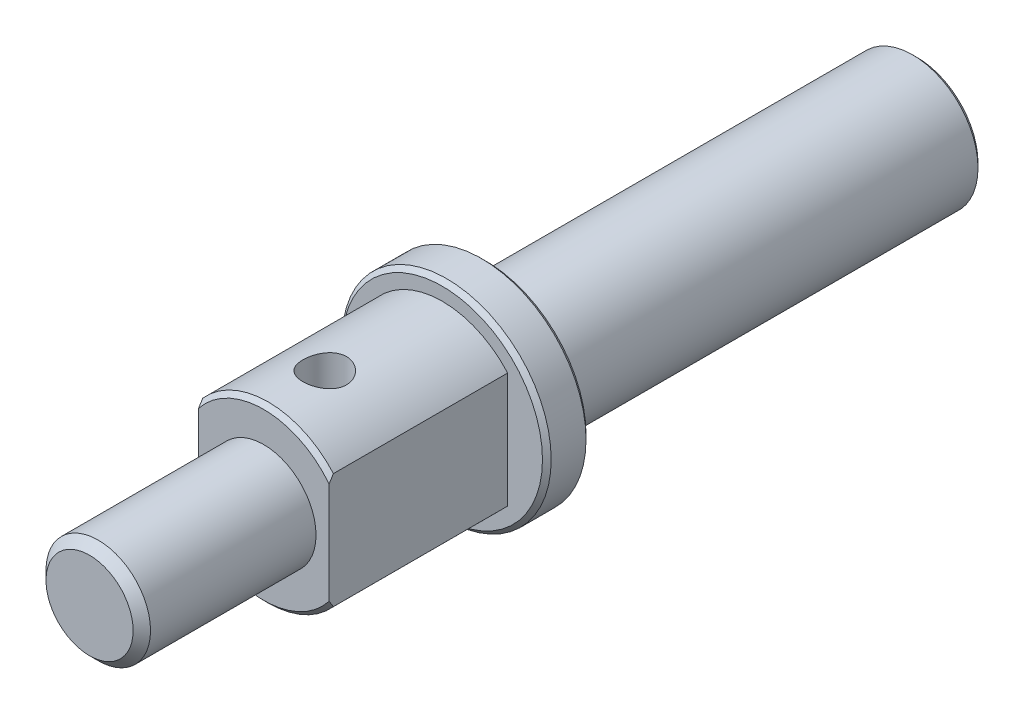
SolidWorks part; units mm, degrees
ref_plane "前视基准面" through (0, 0, 0) normal (0, 0, 1) x (1, 0, 0)
ref_plane "上视基准面" through (0, 0, 0) normal (0, 1, 0) x (1, 0, 0)
ref_plane "右视基准面" through (0, 0, 0) normal (1, 0, 0) x (0, 0, -1)
sketch "草图1" plane through (0, 0, 0) normal (0, 0, 1) x (1, 0, 0)
  circle A0 centre (0, 0) radius 7.5
  dimension "D1" = 15
extrude "凸台-拉伸1" add sketch "草图1" along normal blind 49.5
sketch "草图2" plane through (0, 0, 49.5) normal (0, 0, 1) x (1, 0, 0)
  circle A0 centre (0, 0) radius 12
  dimension "D1" = 24
extrude "凸台-拉伸2" add sketch "草图2" along normal blind 5
sketch "草图3" plane through (0, 0, 54.5) normal (0, 0, 1) x (1, 0, 0)
  circle A0 centre (0, 0) radius 10
  dimension "D1" = 20
extrude "凸台-拉伸3" add sketch "草图3" along normal blind 20.5
sketch "草图4" plane through (0, 0, 75) normal (0, 0, 1) x (1, 0, 0)
  circle A0 centre (0, 0) radius 6
  dimension "D1" = 12
extrude "凸台-拉伸4" add sketch "草图4" along normal blind 20
cosmetic thread "装饰螺纹线1" parameters "D2"=11
hole_wizard "M6 螺纹孔1" positions "草图6" profile "草图5" tap size "M6" standard "Iso"
sketch "草图6" plane through (0, 0, 0) normal (0, 0, -1) x (-1, 0, 0)
  point P0 (0, 0)
sketch "草图5" plane through (0, 0, 0) normal (1, 0, 0) x (0, 1, 0)
  line L0 (0, 0) -> (0, 16.5022)
  line L1 (0, 16.5022) -> (2.5, 15)
  line L2 (2.5, 15) -> (2.5, 0)
  line L5 (2.5, 0) -> (0, 0)
  line L10 (0, 16.5022) -> (-2.5, 15) construction
  line L11 (0, -6.35) -> (0, 107.95) construction
  dimension "螺纹孔钻头直径" = 5
  dimension "螺纹孔钻头深度" = 15
  dimension "导头角度" = 118
cosmetic thread "孔螺蚊线1" parameters "D1"=12, "D2"=6
chamfer "倒角1" distance 0.5 angle 45 3 edges at (12, 0, 54.5) (12, 0, 49.5) (7.5, 0, 0)
chamfer "倒角2" distance 1 angle 45 1 edges at (6, 0, 95)
chamfer "倒角3" distance 0.5 angle 45 1 edges at (10, 0, 75)
sketch "草图7" plane through (0, 0, 0) normal (0, 1, 0) x (1, 0, 0)
  line L0 (0, 0) -> (0, -99.4966) construction
  line L1 (-10, -54.5) -> (10, -54.5) construction
  line L2 (-7.5, -54.5) -> (-33.9603, -54.5)
  line L3 (-7.5, -54.5) -> (-7.5, -80.9728)
  line L4 (-7.5, -80.9728) -> (-33.9603, -80.9728)
  line L5 (-33.9603, -54.5) -> (-33.9603, -80.9728)
  line L7 (7.5, -54.5) -> (26.9987, -54.5)
  line L8 (7.5, -54.5) -> (7.5, -83.2477)
  line L9 (7.5, -83.2477) -> (26.9987, -83.2477)
  line L10 (26.9987, -54.5) -> (26.9987, -83.2477)
  dimension "D1" = 7.5
  dimension "D2" = 15
extrude "切除-拉伸1" cut sketch "草图7" against normal mid plane 104
ref_plane "基准面1" through (0, 10, 0) normal (0, 1, 0) x (1, 0, 0)
hole_wizard "M6 螺纹孔2" positions "草图9" profile "草图8" tap size "M6" standard "Iso" end condition through all
sketch "草图9" plane through (0, 10, 0) normal (0, 1, 0) x (1, 0, 0)
  line L0 (0, -54.5) -> (0, -68) construction
  line L1 (-7.5, -54.5) -> (7.5, -54.5) construction
  point P2 (0, -68)
  dimension "D1" = 13.5
cosmetic thread "孔螺蚊线2" parameters "D2"=6
sketch "草图8" plane through (0, 10, 68) normal (1, 0, 0) x (0, 0, 1)
  line L0 (0, 0) -> (0, 22)
  line L1 (0, 22) -> (2.5, 22)
  line L2 (2.5, 22) -> (2.5, 0)
  line L5 (2.5, 0) -> (0, 0)
  line L11 (0, -6.35) -> (0, 107.95) construction
  dimension "通孔螺纹孔钻头直径" = 5
  dimension "通孔螺纹孔钻头深度" = 22
